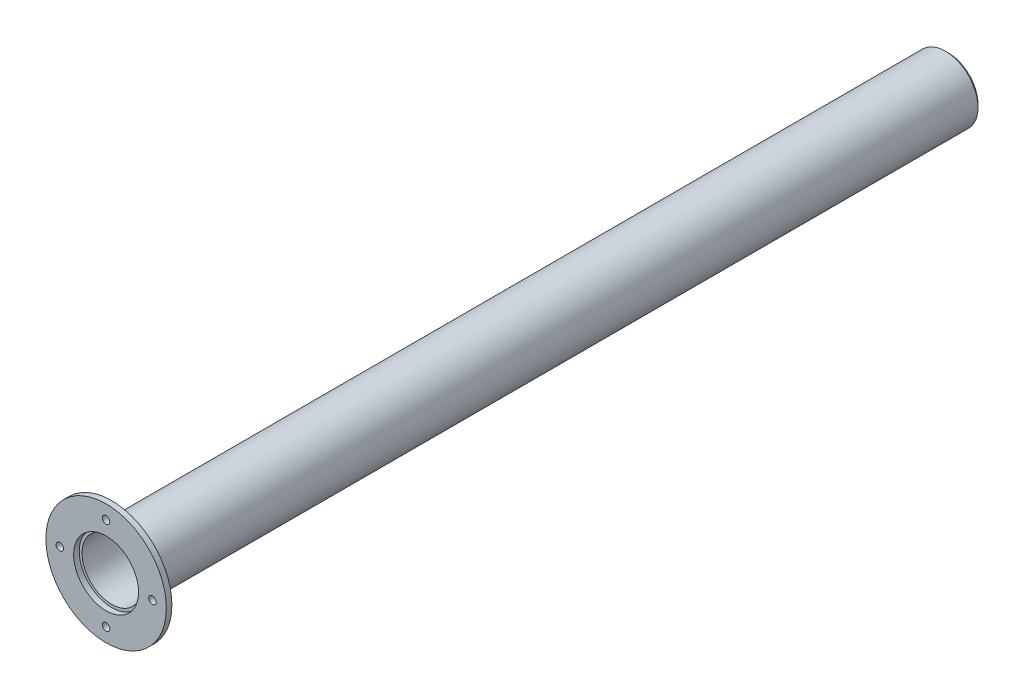
from build123d import *

# Parameters (mm, degrees)
SKETCH1_R                = 35
SKETCH1_R_2              = 32
THIN_EXTRUDE1_DEPTH      = 900
SKETCH3_R                = 32
BOSS_EXTRUDE1_DEPTH      = 3
SKETCH4_R                = 65
SKETCH4_R_2              = 35
BOSS_EXTRUDE2_DEPTH      = 6
SKETCH6_W                = 4
SKETCH6_H                = 6.001
F_8_0_8_HOLE1_AT_2_COUNT = 2
F_8_0_8_HOLE1_AT_2_PITCH = 70.710678119
F_8_0_8_HOLE1_AT_3_COUNT = 2
F_8_0_8_HOLE1_AT_3_PITCH = 100
F_8_0_8_HOLE1_AT_4_COUNT = 2
F_8_0_8_HOLE1_AT_4_PITCH = 70.710678119


with BuildPart() as part:
    # Sketch1 → Thin Extrude1 (new body)
    with BuildSketch(Plane.XY):
        Circle(SKETCH1_R)
        Circle(SKETCH1_R_2, mode=Mode.SUBTRACT)
    extrude(amount=THIN_EXTRUDE1_DEPTH)


with BuildPart() as body_2:
    # Sketch3 → Boss-Extrude1 (new body)
    with BuildSketch(Plane(origin=(0, 0, 0), x_dir=(-1, 0, 0), z_dir=(0, 0, -1))):
        Circle(SKETCH3_R)
    extrude(amount=BOSS_EXTRUDE1_DEPTH)


with BuildPart() as body_3:
    # Sketch4 → Boss-Extrude2 (new body)
    with BuildSketch(Plane.XY.offset(900)):
        Circle(SKETCH4_R)
        Circle(SKETCH4_R_2, mode=Mode.SUBTRACT)
    extrude(amount=BOSS_EXTRUDE2_DEPTH)

    # Sketch6 → Ø8.0 (8) Hole1 (revolve, cut)
    with BuildSketch(Plane(origin=(0, 50, 906), x_dir=(0, -1, 0), z_dir=(1, 0, 0))):
        with Locations((2, 3.0005)):
            Rectangle(SKETCH6_W, SKETCH6_H)
    f_8_0_8_hole1 = revolve(axis=Axis((0, 50, 912.35), (0, 0, -1)), mode=Mode.SUBTRACT)

    # Ø8.0 (8) Hole1 at 2: Ø8.0 (8) Hole1 ×2
    with Locations(*[Vector(-0.7071067811865476, -0.7071067811865476, 0) * (i * F_8_0_8_HOLE1_AT_2_PITCH) for i in range(1, F_8_0_8_HOLE1_AT_2_COUNT)]):
        add(f_8_0_8_hole1, mode=Mode.SUBTRACT)

    # Ø8.0 (8) Hole1 at 3: Ø8.0 (8) Hole1 ×2
    with Locations(*[(0, -i * F_8_0_8_HOLE1_AT_3_PITCH, 0) for i in range(1, F_8_0_8_HOLE1_AT_3_COUNT)]):
        add(f_8_0_8_hole1, mode=Mode.SUBTRACT)

    # Ø8.0 (8) Hole1 at 4: Ø8.0 (8) Hole1 ×2
    with Locations(*[Vector(0.7071067811865476, -0.7071067811865476, 0) * (i * F_8_0_8_HOLE1_AT_4_PITCH) for i in range(1, F_8_0_8_HOLE1_AT_4_COUNT)]):
        add(f_8_0_8_hole1, mode=Mode.SUBTRACT)


solid = Compound([part.part, body_2.part, body_3.part])
